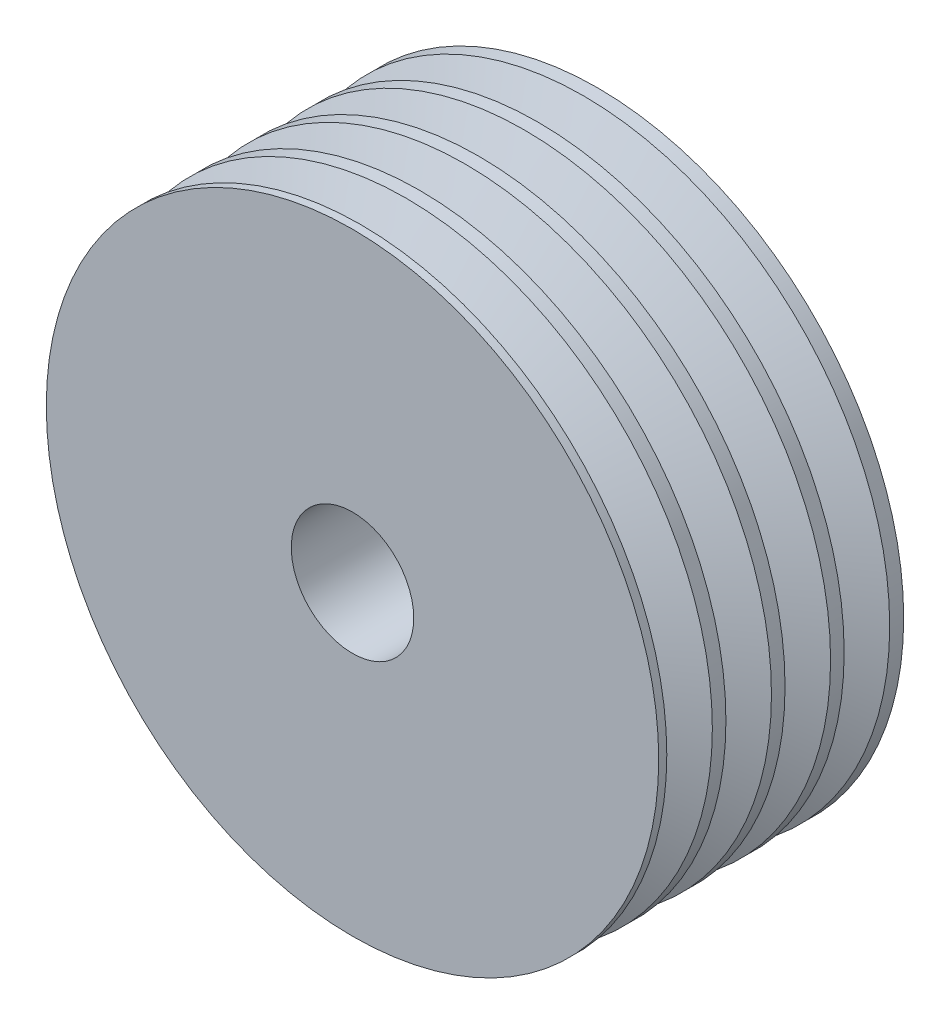
SolidWorks part; units mm, degrees
ref_plane "前视基准面" through (0, 0, 0) normal (0, 0, 1) x (1, 0, 0)
ref_plane "上视基准面" through (0, 0, 0) normal (0, 1, 0) x (1, 0, 0)
ref_plane "右视基准面" through (0, 0, 0) normal (1, 0, 0) x (0, 0, -1)
sketch "草图1" plane through (0, 0, 0) normal (0, 0, 1) x (1, 0, 0)
  circle A0 centre (0, 0) radius 75
  circle A1 centre (0, 0) radius 15
  dimension "D1" = 150
  dimension "D2" = 30
extrude "凸台-拉伸1" add sketch "草图1" along normal blind 60
sketch "草图2" plane through (0, 0, 0) normal (0, 1, 0) x (1, 0, 0)
  line L1 (-75, 0) -> (-75, -60) construction
  line L5 (0, 0) -> (0, 11.8359) construction
  line L6 (-75, -46.8663) -> (-75, -58.0223)
  line L7 (-64.2634, -51.5728) -> (-75, -46.8663)
  line L8 (-64.2634, -52.3072) -> (-64.2634, -51.5728)
  line L9 (-75, -58.0223) -> (-64.2634, -52.3072)
  line L10 (75, 0) -> (-75, 0) construction
  line L11 (-75, 0) -> (-75, -60) construction
  line L12 (-75, -32.3866) -> (-75, -43.5426)
  line L13 (-75, -43.5426) -> (-64.2634, -37.8275)
  line L14 (-64.2634, -37.0931) -> (-75, -32.3866)
  line L15 (-64.2634, -37.8275) -> (-64.2634, -37.0931)
  line L16 (-75, -17.9069) -> (-75, -29.0629)
  line L17 (-75, -29.0629) -> (-64.2634, -23.3479)
  line L18 (-64.2634, -22.6134) -> (-75, -17.9069)
  line L19 (-64.2634, -23.3479) -> (-64.2634, -22.6134)
  line L20 (-75, -3.4272) -> (-75, -14.5832)
  line L21 (-75, -14.5832) -> (-64.2634, -8.8682)
  line L22 (-64.2634, -8.1337) -> (-75, -3.4272)
  line L23 (-64.2634, -8.8682) -> (-64.2634, -8.1337)
  dimension "D1" = 4
sketch "草图3" plane through (0, 0, 0) normal (0, 1, 0) x (1, 0, 0)
  line L0 (0, 0) -> (0, 11.3879) construction
  line L1 (75, 0) -> (-75, 0) construction
revolve "切除-旋转2" cut sketch "草图2" angle 360 about L5
